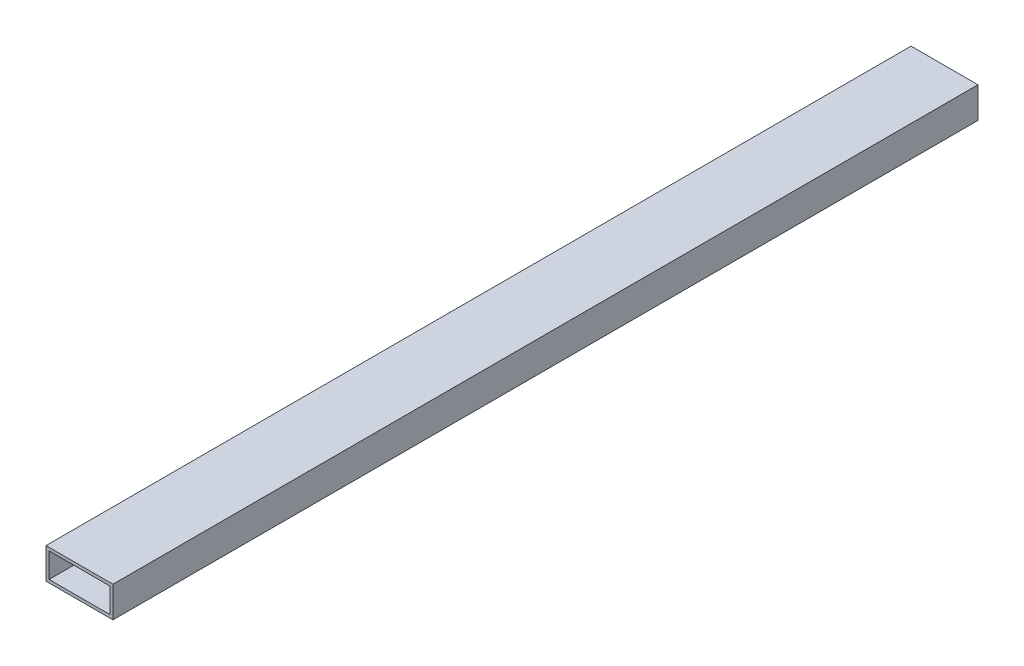
from build123d import *

# Parameters (mm, degrees)
SKETCH1_W           = 65
SKETCH1_H           = 30
BOSS_EXTRUDE1_DEPTH = 840
SKETCH2_W           = 59
SKETCH2_H           = 24
CUT_EXTRUDE1_DEPTH  = 950


with BuildPart() as part:
    # Sketch1 → Boss-Extrude1 (new body)
    with BuildSketch(Plane.XY):
        with Locations((-8.040751589, 24.808027615)):
            Rectangle(SKETCH1_W, SKETCH1_H)
    extrude(amount=BOSS_EXTRUDE1_DEPTH)

    # Sketch2 → Cut-Extrude1 (cut)
    with BuildSketch(Plane.XY.offset(840)):
        with Locations((-8.040751589, 24.808027615)):
            Rectangle(SKETCH2_W, SKETCH2_H)
    extrude(amount=-CUT_EXTRUDE1_DEPTH, mode=Mode.SUBTRACT)


solid = part.part
